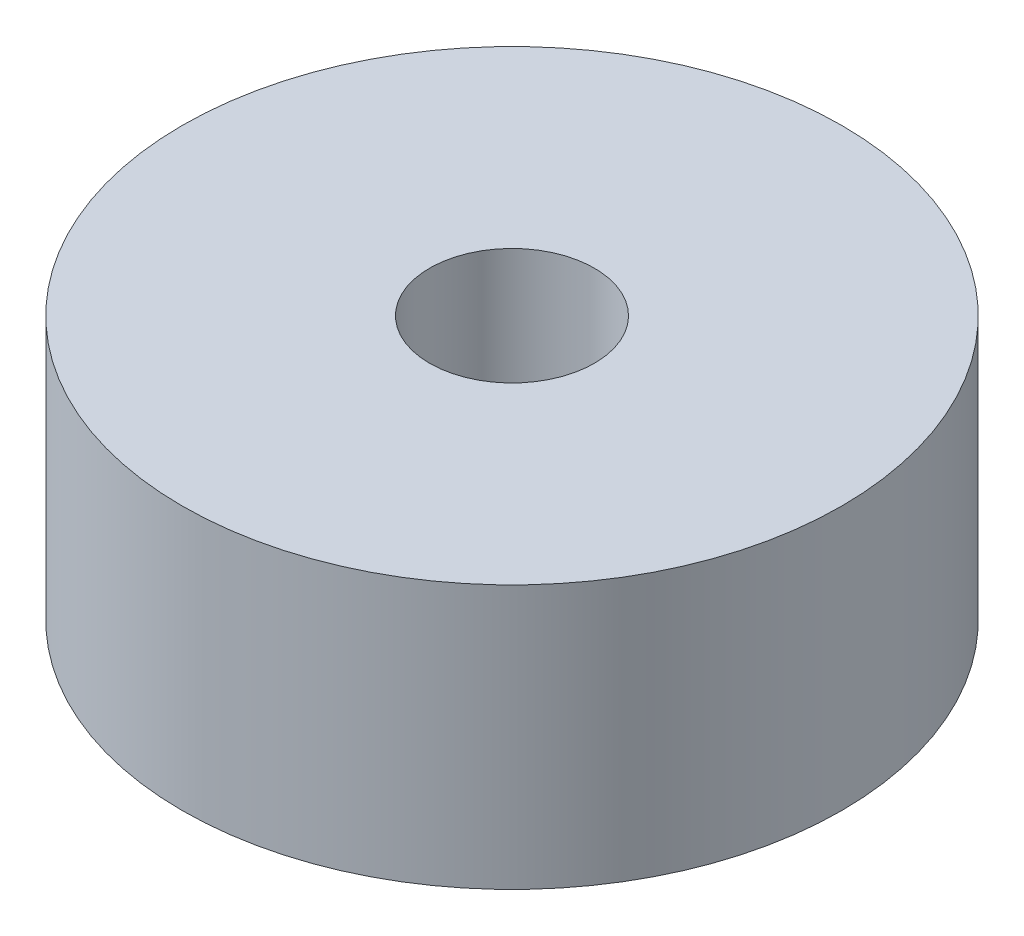
SolidWorks part; units mm, degrees
ref_plane "Front Plane" through (0, 0, 0) normal (0, 0, 1) x (1, 0, 0)
ref_plane "Top Plane" through (0, 0, 0) normal (0, 1, 0) x (1, 0, 0)
ref_plane "Right Plane" through (0, 0, 0) normal (1, 0, 0) x (0, 0, -1)
sketch "Sketch1" plane through (0, 0, 0) normal (0, 1, 0) x (1, 0, 0)
  circle A0 centre (0, 0) radius 2.5
  circle A1 centre (0, 0) radius 10
  dimension "D1" = 20
  dimension "D2" = 5
extrude "Boss-Extrude1" add sketch "Sketch1" along normal blind 8
